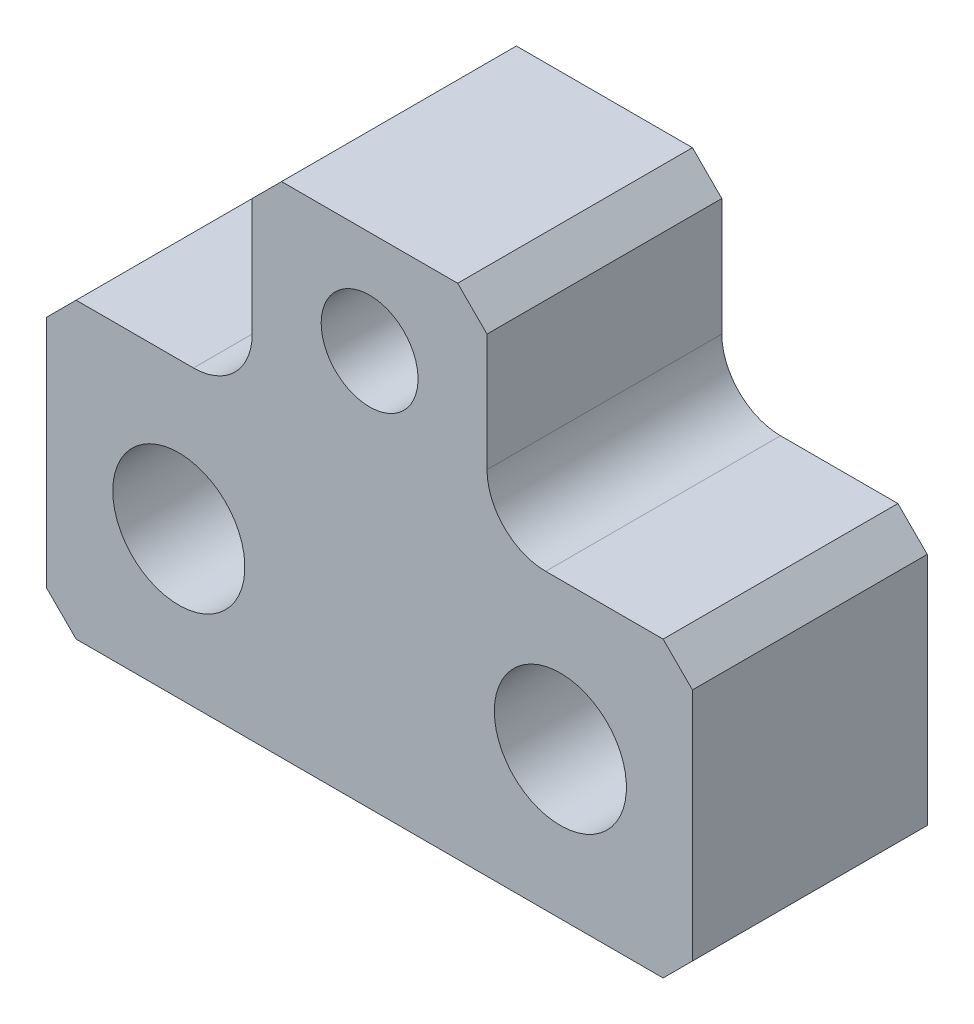
from build123d import *

# Parameters (mm, degrees)
SKETCH1_W                                            = 22
SKETCH1_H                                            = 10
BOSS_EXTRUDE1_DEPTH                                  = 8
CBORE_FOR_M4_HEXAGON_SOCKET_HEAD_CAP_SCR_D           = 4.5
CBORE_FOR_M4_HEXAGON_SOCKET_HEAD_CAP_SCR_CBORE_D     = 8
CBORE_FOR_M4_HEXAGON_SOCKET_HEAD_CAP_SCR_CBORE_DEPTH = 4.6
SKETCH4_W                                            = 8
SKETCH4_H                                            = 7
BOSS_EXTRUDE2_DEPTH                                  = 8
M4_TAPPED_HOLE1_D                                    = 3.3
FILLET1_R                                            = 2
CHAMFER1_SIZE                                        = 1


with BuildPart() as part:
    # Sketch1 → Boss-Extrude1 (new body)
    with BuildSketch(Plane.XY):
        Rectangle(SKETCH1_W, SKETCH1_H)
    extrude(amount=BOSS_EXTRUDE1_DEPTH)

    # CBORE for M4 Hexagon socket head cap screws1 (through all)
    with Locations(Plane(origin=(0, 0, 0), x_dir=(-1, 0, 0), z_dir=(0, 0, -1))):
        with Locations((-6.5, 0), (6.5, 0)):
            CounterBoreHole(CBORE_FOR_M4_HEXAGON_SOCKET_HEAD_CAP_SCR_D / 2, CBORE_FOR_M4_HEXAGON_SOCKET_HEAD_CAP_SCR_CBORE_D / 2, CBORE_FOR_M4_HEXAGON_SOCKET_HEAD_CAP_SCR_CBORE_DEPTH)

    # Sketch4 → Boss-Extrude2 (add)
    with BuildSketch(Plane(origin=(0, 0, 0), x_dir=(-1, 0, 0), z_dir=(0, 0, -1))):
        with Locations((0, 8.5)):
            Rectangle(SKETCH4_W, SKETCH4_H)
    extrude(amount=-BOSS_EXTRUDE2_DEPTH)

    # M4 Tapped Hole1 (through all)
    with Locations(Plane(origin=(0, 0, 0), x_dir=(-1, 0, 0), z_dir=(0, 0, -1))):
        with Locations((0, 8.5)):
            Hole(M4_TAPPED_HOLE1_D / 2)

    # Fillet1
    fillet1_edges = [part.edges().sort_by_distance(p)[0] for p in [
        (4, 5, 4),
        (-4, 5, 4),
    ]]
    fillet(fillet1_edges, radius=FILLET1_R)

    # Chamfer1
    chamfer1_edges = [part.edges().sort_by_distance(p)[0] for p in [
        (4, 12, 4),
        (-4, 12, 4),
        (11, -5, 4),
        (-11, -5, 4),
        (-11, 5, 4),
        (11, 5, 4),
    ]]
    chamfer(chamfer1_edges, length=CHAMFER1_SIZE)


solid = part.part
